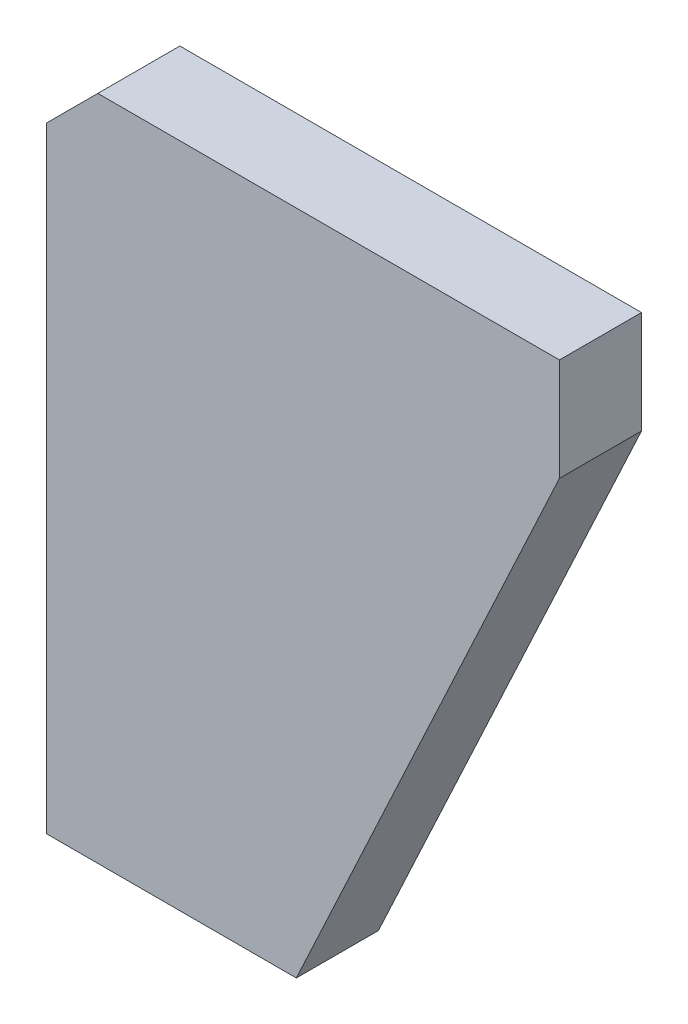
from build123d import *

# Parameters (mm, degrees)
BOSS_EXTRUDE1_DEPTH = 8
CHAMFER1_SIZE       = 5


with BuildPart() as part:
    # Sketch1 → Boss-Extrude1 (new body)
    with BuildSketch(Plane.XY):
        Polygon((50, 65), (0, 65), (0, 0), (24.353078801, 0), (50, 55), align=None)
    extrude(amount=BOSS_EXTRUDE1_DEPTH)

    # Chamfer1
    chamfer1_edges = [part.edges().sort_by_distance(p)[0] for p in [
        (0, 65, 4),
    ]]
    chamfer(chamfer1_edges, length=CHAMFER1_SIZE)


solid = part.part
